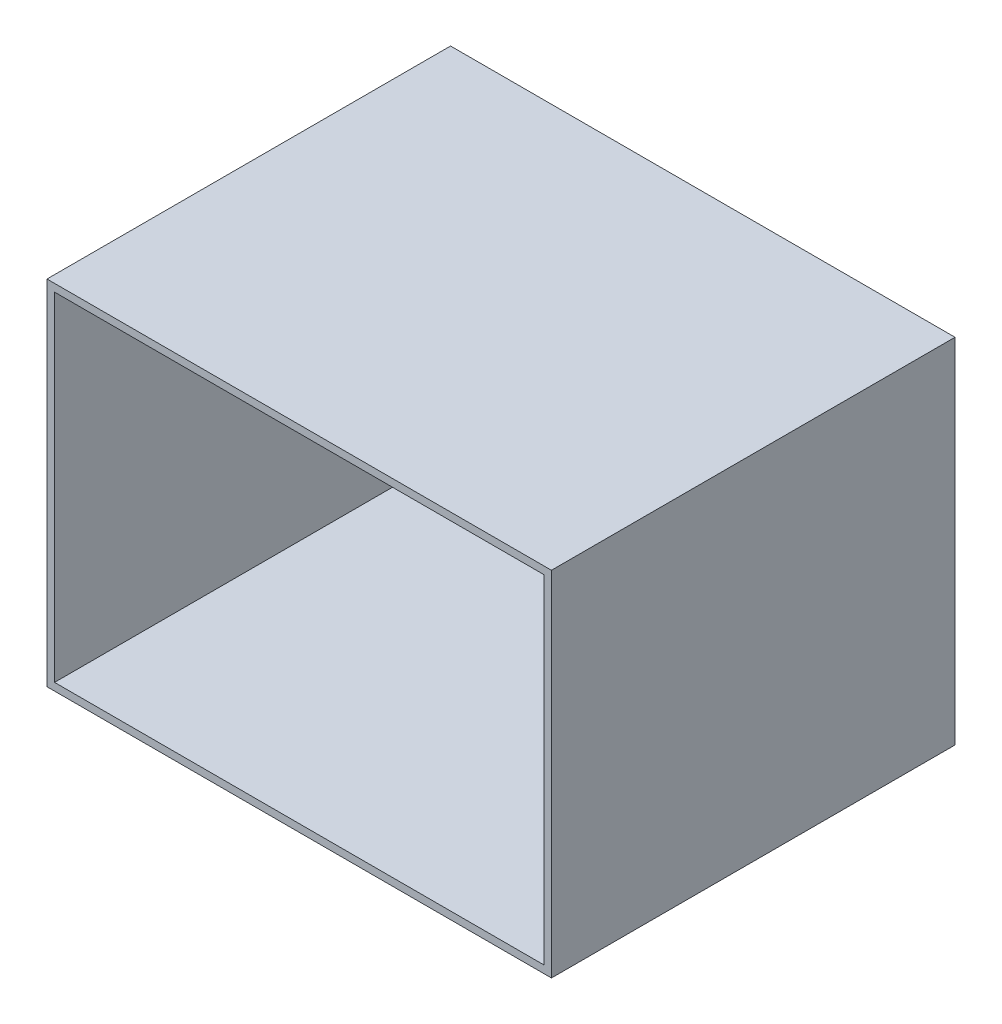
SolidWorks part; units mm, degrees
ref_plane "前视基准面" through (0, 0, 0) normal (0, 0, 1) x (1, 0, 0)
ref_plane "上视基准面" through (0, 0, 0) normal (0, 1, 0) x (1, 0, 0)
ref_plane "右视基准面" through (0, 0, 0) normal (1, 0, 0) x (0, 0, -1)
other "Configuration Table"
sketch "草图1" plane through (0, 0, 0) normal (0, 0, 1) x (1, 0, 0)
  line L0 (-100, -70) -> (100, -70)
  line L1 (100, -70) -> (100, 70)
  line L2 (100, 70) -> (-100, 70)
  line L3 (-100, 70) -> (-100, -70)
  line L4 (-97, -67) -> (97, -67)
  line L5 (97, -67) -> (97, 67)
  line L6 (97, 67) -> (-97, 67)
  line L7 (-97, 67) -> (-97, -67)
  point P0 (0, 0)
  dimension "D1" = 3
  dimension "D2" = 100
  dimension "D3" = 197
  dimension "D4" = 200
  dimension "D5" = 3
  dimension "D6" = 70
  dimension "D7" = 137
  dimension "D8" = 140
extrude "凸台-拉伸1" add sketch "草图1" against normal mid plane 160
